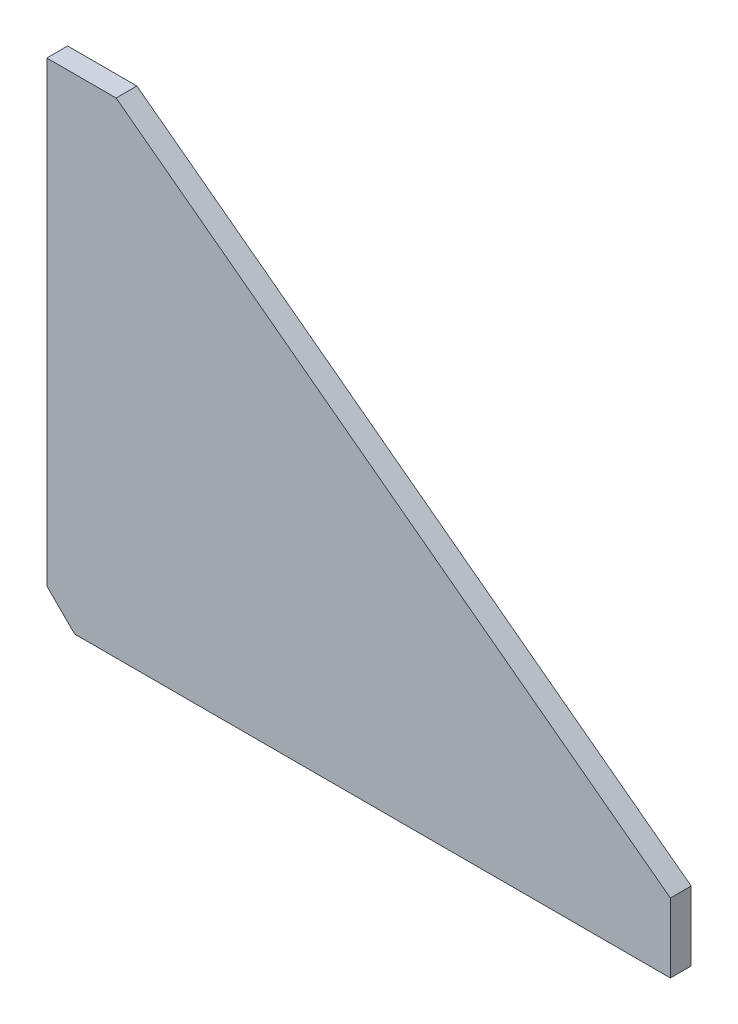
from build123d import *

# Parameters (mm, degrees)
BOSS_EXTRUDE1_DEPTH = 1.5


with BuildPart() as part:
    # Sketch1 → Boss-Extrude1 (new body)
    with BuildSketch(Plane.XY):
        Polygon((-17.5, 17.5), (22.5, -12.5), (22.5, -17.5), (-20.5, -17.5), (-22.5, -15.5), (-22.5, 17.5), align=None)
    extrude(amount=BOSS_EXTRUDE1_DEPTH)


solid = part.part
